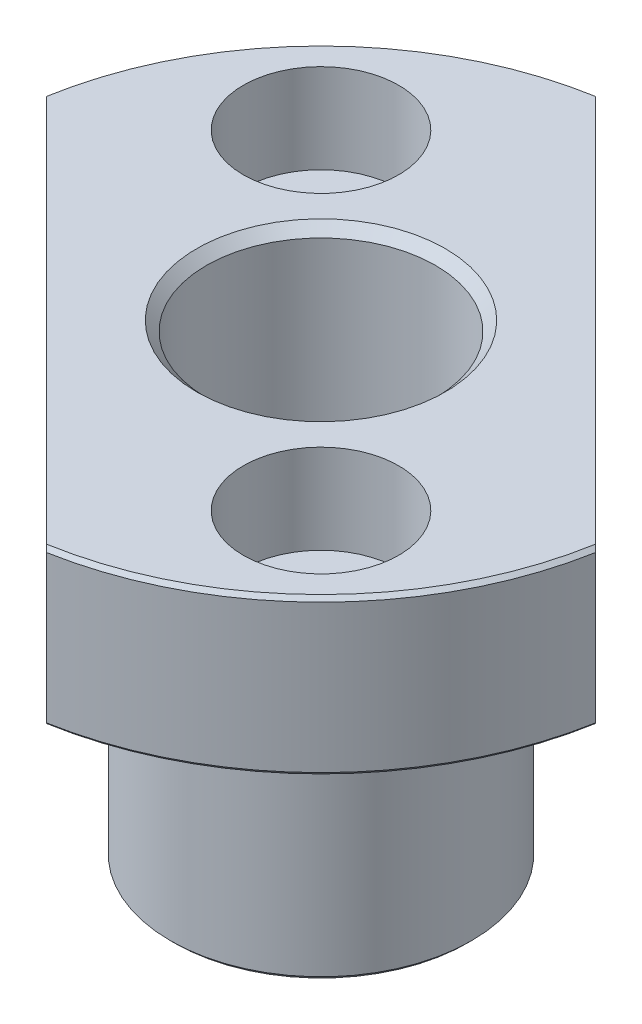
SolidWorks part; units mm, degrees
material "AISI 类型 316L 不锈钢"
ref_plane "Front Plane" through (0, 0, 0) normal (0, 0, 1) x (1, 0, 0)
ref_plane "Top Plane" through (0, 0, 0) normal (0, 1, 0) x (1, 0, 0)
ref_plane "Right Plane" through (0, 0, 0) normal (1, 0, 0) x (0, 0, -1)
sketch "Sketch2" plane through (0, 0, 0) normal (0, 0, 1) x (1, 0, 0)
  line L0 (0, 0) -> (0, 24) construction
  line L1 (0, 24) -> (-17.5, 24)
  line L2 (-17.5, 24) -> (-17.5, 16)
  line L3 (-17.5, 16) -> (-7.75, 16)
  line L4 (-7.75, 16) -> (-7.75, 0)
  line L5 (-7.75, 0) -> (0, 0)
  line L6 (0, 0) -> (0, 24)
  dimension "D1" = 35
  dimension "D2" = 15.5
  dimension "D3" = 16
  dimension "D4" = 8
revolve "Revolve1" add sketch "Sketch2" angle 360 about L0
hole_wizard "G1/4 Tapped Hole1" positions "3DSketch1" profile "Sketch4" tap size "G1/4" standard "GB" end condition up to next
sketch3d "3DSketch1"
  line L0 (0, 24, 0) -> (0, 16, 0) construction
  point P0 (0, 24, 0)
sketch "Sketch4" plane through (0, 24, 0) normal (1, 0, 0) x (0, 0, 1)
  line L0 (0, 0) -> (0, 24)
  line L1 (0, 24) -> (5.9, 24)
  line L2 (5.9, 24) -> (5.9, 0)
  line L5 (5.9, 0) -> (0, 0)
  line L11 (0, -6.35) -> (0, 107.95) construction
  dimension "通孔螺纹孔钻头直径" = 11.8
  dimension "通孔螺纹孔钻头深度" = 24
cosmetic thread "Cosmetic Thread 1" parameters "D2"=13.157
sketch "Sketch5" plane through (0, 24, 0) normal (0, 1, 0) x (1, 0, 0)
  line L0 (0, 12) -> (0, -12) construction
  line L1 (12, 0) -> (-12, 0) construction
  line L2 (0, 0) -> (-8.4853, 8.4853) construction
  line L3 (0, 0) -> (8.4853, -8.4853) construction
  circle A0 centre (0, 0) radius 12 construction
  dimension "D1" = 24
  dimension "D2" = 45
hole_wizard "Hole Size (% based on) Socket Head Cap Screw Type 1" positions "3DSketch2" profile "Sketch6" counterbore size "M4" standard "GB" end condition up to next
sketch3d "3DSketch2"
  point P13 (-8.4853, 24, -8.4853)
  point P16 (8.4853, 24, 8.4853)
sketch "Sketch6" plane through (-8.4853, 24, -8.4853) normal (1, 0, 0) x (0, 0, 1)
  line L0 (0, 0) -> (0, 8)
  line L1 (0, 8) -> (2.4, 8)
  line L3 (2.4, 8) -> (2.4, 4.6)
  line L4 (2.4, 4.6) -> (4, 4.6)
  line L5 (4, 4.6) -> (4, 0)
  line L7 (4, 0) -> (0, 0)
  line L11 (0, -6.35) -> (0, 107.95) construction
  dimension "通孔孔直径" = 4.8
  dimension "通孔孔深度" = 8
  dimension "柱形沉头孔直径" = 8
  dimension "柱形沉头孔深度" = 4.6
fillet "Fillet1" radius 0.2 1 edges at (0, 16, -7.75)
chamfer "Chamfer1" distance 0.2 angle 45 3 edges at (0, 0, -7.75) (0, 24, -17.5) (0, 16, -17.5)
chamfer "Chamfer2" distance 0.5 angle 45 2 edges at (0, 0, 5.9) (0, 24, 5.9)
sketch "Sketch7" plane through (0, 24, 0) normal (0, 1, 0) x (1, 0, 0)
  line L0 (0, 0) -> (12.2329, 12.2329) construction
  line L1 (0, 0) -> (17.3, 0) construction
  line L2 (-3.084, 17.2261) -> (17.2261, -3.084)
  line L3 (0, 0) -> (12.2329, -12.2329) construction
  line L4 (0, 12) -> (0, -12) construction
  line L5 (-17.2261, 3.084) -> (3.084, -17.2261)
  circle A0 centre (0, 0) radius 17.3 construction
  circle A1 centre (0, 0) radius 17.5 construction
  circle A2 centre (0, 0) radius 17.5
  point P9 (7.0711, 7.0711)
  circle M7 centre (0, 0) radius 17.3
  dimension "D1" = 45
  dimension "D2" = 45
  dimension "D3" = 10
extrude "Cut-Extrude1" cut sketch "Sketch7" against normal through all contours L5 M7 | L2 M7 | L5 A2 M7 | L2 A2 M7
